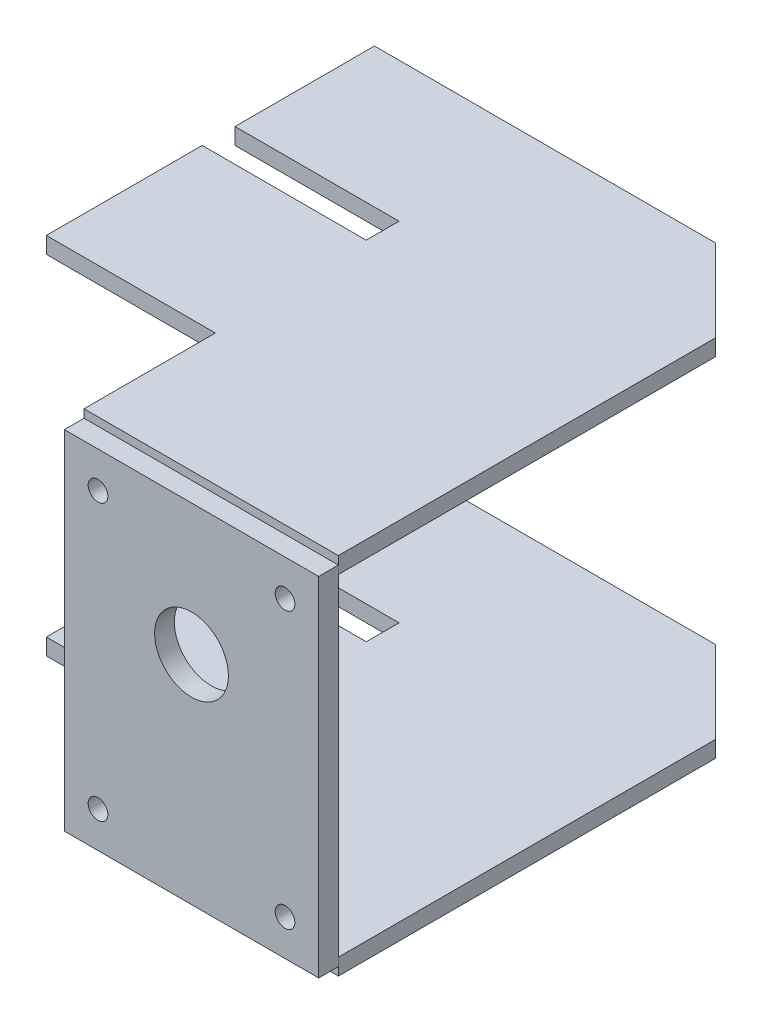
SolidWorks part; units mm, degrees
material "K"
ref_plane "Front" through (0, 0, 0) normal (0, 0, 1) x (1, 0, 0)
ref_plane "Top" through (0, 0, 0) normal (0, 1, 0) x (1, 0, 0)
ref_plane "Right" through (0, 0, 0) normal (1, 0, 0) x (0, 0, -1)
sketch "Sketch1" plane through (0, 0, 0) normal (0, 0, 1) x (1, 0, 0)
  line L1 (77.5, -106) -> (-77.5, -106)
  line L2 (77.5, -106) -> (77.5, 106)
  line L3 (77.5, 106) -> (-77.5, 106)
  line L4 (-77.5, -106) -> (-77.5, 106)
  line L5 (0, 106) -> (0, -106) construction
  line L6 (77.5, 0) -> (-77.5, 0) construction
  point P0 (0, 0)
  dimension "D1" = 155
  dimension "D2" = 212
extrude "Boss-Extrude1" add sketch "Sketch1" along normal blind 12
sketch "Sketch2" plane through (0, 0, 0) normal (0, 0, -1) x (-1, 0, 0)
  line L0 (0, 106) -> (0, -106) construction
  line L1 (-77.5, 106) -> (77.5, 106) construction
  line L2 (77.5, -106) -> (-77.5, -106) construction
sketch "Sketch3" plane through (0, 0, 0) normal (0, 0, -1) x (-1, 0, 0)
  line L1 (57, -84) -> (-57, -84) construction
  line L2 (57, -84) -> (57, 84) construction
  line L3 (57, 84) -> (-57, 84) construction
  line L4 (-57, -84) -> (-57, 84) construction
  line L5 (0, 84) -> (0, -84) construction
  line L6 (57, 0) -> (-57, 0) construction
  line L7 (0, 106) -> (0, -106) construction
  dimension "D1" = 168
  dimension "D2" = 114
hole_wizard "Ø12.0 (12) Hole1" positions "Sketch5" profile "Sketch4" hole size "Ø12.0" standard "GB" end condition up to next
sketch "Sketch5" plane through (0, 0, 0) normal (0, 0, -1) x (-1, 0, 0)
  point P0 (-57, 84)
  point P3 (57, 84)
  point P6 (-57, -84)
  point P9 (57, -84)
sketch "Sketch4" plane through (57, 84, 0) normal (1, 0, 0) x (0, 1, 0)
  line L0 (0, 0) -> (0, 12)
  line L1 (0, 12) -> (6, 12)
  line L2 (6, 12) -> (6, 0)
  line L5 (6, 0) -> (0, 0)
  line L11 (0, -6.35) -> (0, 107.95) construction
  dimension "通孔孔直径" = 12
  dimension "通孔孔深度" = 12
sketch "Sketch8" plane through (0, 106, 0) normal (0, 1, 0) x (1, 0, 0)
  line L3 (77.5, 0) -> (-77.5, 0)
  line L6 (0, 0) -> (0, 167.9322) construction
  line L7 (77.5, 0) -> (77.5, 280)
  line L8 (-180.5, 280) -> (-180.5, 80)
  line L9 (77.5, 280) -> (-180.5, 280)
  line L10 (-77.5, 80) -> (-180.5, 80)
  line L11 (-77.5, 0) -> (-77.5, 80)
  dimension "D1" = 200
  dimension "D2" = 258
  dimension "D3" = 80
extrude "Boss-Extrude2" add sketch "Sketch8" along normal mid plane 10 separate body
chamfer "Chamfer1" distance 50 angle 45 1 edges at (77.5, 106, -280)
mirror "Mirror1" about plane through (0, 0, 0) normal (0, 1, 0) of bodies 104
sketch "Sketch9" plane through (0, 0, 0) normal (0, 0, -1) x (-1, 0, 0)
  circle A0 centre (0, 26) radius 22.5
  dimension "D1" = 45
extrude "Cut-Extrude1" cut sketch "Sketch9" against normal up to next (12 mm away)
sketch "Sketch10" plane through (0, 111, 0) normal (0, 1, 0) x (1, 0, 0)
  line L0 (-180.5, 280) -> (-180.5, 80) construction
  line L1 (-180.5, 195) -> (-80.5, 195)
  line L2 (-180.5, 195) -> (-180.5, 175)
  line L3 (-180.5, 175) -> (-80.5, 175)
  line L4 (-80.5, 195) -> (-80.5, 175)
  line L5 (-180.5, 80) -> (-77.5, 80) construction
  dimension "D1" = 20
  dimension "D2" = 95
  dimension "D3" = 100
extrude "Cut-Extrude2" cut sketch "Sketch10" against normal through all
equation "\"零件重量\"= IIF ( \"SW-质量\" > 100 , int ( \"SW-质量\" ) , \"SW-质量\" )"
